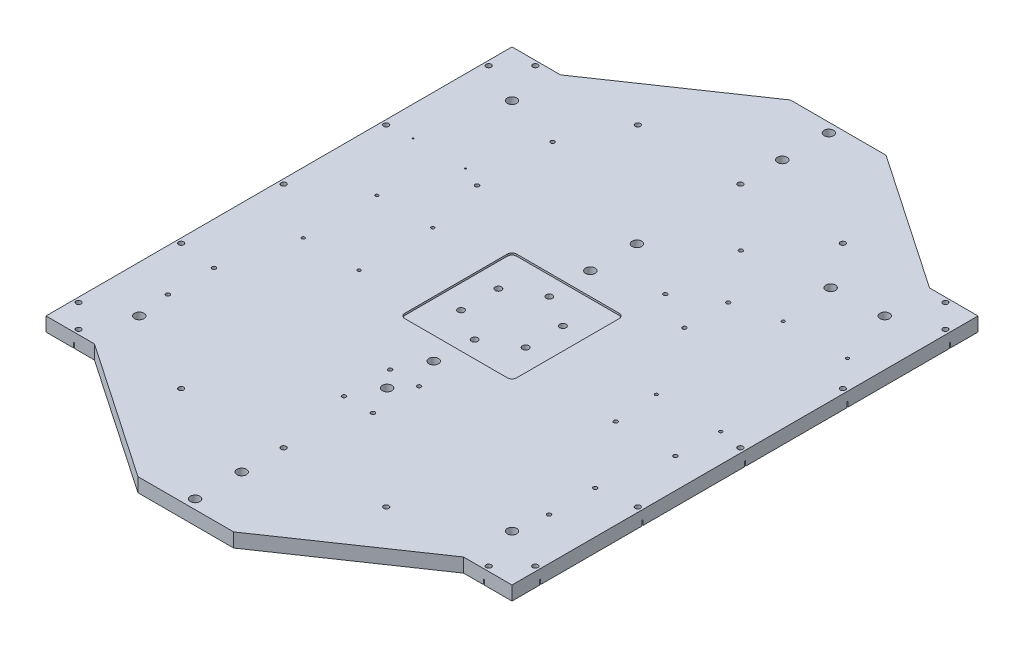
from build123d import *

# Parameters (mm, degrees)
SKETCH_5_W                     = 500
SKETCH_5_H                     = 500
EXTRUDE_1_DEPTH                = 15
EXTRUDE_2_DEPTH                = 60
EXTRUDE_3_DEPTH                = 60
HOLE_WIZARD_M8_1_D             = 6.8
HOLE_WIZARD_10_2_10_2_2_D      = 10.2
HOLE_WIZARD_M5_2_AT_2_COUNT    = 2
HOLE_WIZARD_M5_2_AT_2_PITCH    = 20
HOLE_WIZARD_M5_2_AT_3_COUNT    = 2
HOLE_WIZARD_M5_2_AT_3_PITCH    = 44.72135955
HOLE_WIZARD_M5_2_AT_4_COUNT    = 2
HOLE_WIZARD_M5_2_AT_4_PITCH    = 40
HOLE_WIZARD_M5_1_AT_2_COUNT    = 2
HOLE_WIZARD_M5_1_AT_2_PITCH    = 20
HOLE_WIZARD_M5_1_AT_3_COUNT    = 2
HOLE_WIZARD_M5_1_AT_3_PITCH    = 44.72135955
HOLE_WIZARD_M5_1_AT_4_COUNT    = 2
HOLE_WIZARD_M5_1_AT_4_PITCH    = 40
HOLE_WIZARD_10_2_10_2_1_D      = 10.2
HOLE_WIZARD_M5_3_D             = 4.2
HOLE_WIZARD_M5_4_D             = 4.2
HOLE_WIZARD_M4_1_D             = 3.3
HOLE_WIZARD_M2_1_D             = 1.6
HOLE_WIZARD_M12_3_D            = 10.2
HOLE_WIZARD_M3_5_1_D           = 2.9
HOLE_WIZARD_M3_5_1_DEPTH       = 10
SKETCH_47_W                    = 120
SKETCH_47_H                    = 120
CUT_EXTRUDE_1_DEPTH            = 2
CUT_EXTRUDE_2_DEPTH            = 60
CUT_EXTRUDE_3_DEPTH            = 460.292934847
HOLE_WIZARD_M5_1_2_D           = 5.5
HOLE_WIZARD_M5_1_2_CBORE_D     = 10.1
HOLE_WIZARD_M5_1_2_CBORE_DEPTH = 5.4
FILLET_1_R                     = 5


with BuildPart() as part:
    # 草图5 → 凸台-拉伸1 (new body)
    with BuildSketch(Plane(origin=(0, 0, 0), x_dir=(1, 0, 0), z_dir=(0, 1, 0))):
        Polygon((0, 385), (-198, 250), (198, 250), align=None)
        Rectangle(SKETCH_5_W, SKETCH_5_H)
        Polygon((198, -250), (-198, -250), (0, -385), align=None)
    extrude(amount=EXTRUDE_1_DEPTH)

    # 草图6 → 凸台-拉伸2 (add)
    with BuildSketch(Plane(origin=(0, 15, 0), x_dir=(1, 0, 0), z_dir=(0, 1, 0))):
        Polygon((198, 250), (0, 385), (-198, 250), (-250, 250), (-250, -250), (-198, -250), (0, -385), (198, -250), (250, -250), (250, 250), align=None)
        Polygon((-240, 240), (-240, -240), (-194.915297392, -240), (0, -372.896793677), (194.915297392, -240), (240, -240), (240, 240), (194.915297392, 240), (0, 372.896793677), (-194.915297392, 240), align=None, mode=Mode.SUBTRACT)
    extrude(amount=EXTRUDE_2_DEPTH)

    # 草图16 → 凸台-拉伸3 (add)
    with BuildSketch(Plane(origin=(0, 15, 0), x_dir=(1, 0, 0), z_dir=(0, 1, 0))):
        Polygon((180.248630726, -250), (194.915297392, -240), (-194.915297392, -240), (-180.248630726, -250), align=None)
        Polygon((-180.248630726, 250), (-194.915297392, 240), (194.915297392, 240), (180.248630726, 250), align=None)
    extrude(amount=EXTRUDE_3_DEPTH)

    # M8 螺纹孔1 (through all)
    with Locations(Plane(origin=(0, 15, -40), x_dir=(0, 0, 1), z_dir=(0, 1, 0))):
        with Locations((0, 0), (20, -34.641016151), (20, 34.641016151), (60, 34.641016151), (60, -34.641016151), (80, 0)):
            Hole(HOLE_WIZARD_M8_1_D / 2)

    # Ø10.2 (10.2) 直径孔2 (through all)
    with Locations(Plane(origin=(0, 15, -290), x_dir=(0, 0, 1), z_dir=(0, 1, 0))):
        with Locations((0, 0), (-50, 0), (156, 0), (206, 0)):
            hole_wizard_10_2_10_2_2 = Hole(HOLE_WIZARD_10_2_10_2_2_D / 2)

    # 镜向1: Ø10.2 (10.2) 直径孔2 across plane
    add(hole_wizard_10_2_10_2_2.mirror(Plane.XY), mode=Mode.SUBTRACT)

    # 草图22 → M5 螺纹孔2 (revolve, cut)
    with BuildSketch(Plane(origin=(214, 57.5, 250), x_dir=(0, -1, 0), z_dir=(1, 0, 0))):
        Polygon((0, 0), (0, 15.2618073), (2.1, 14), (2.1, 0), align=None)
    hole_wizard_m5_2 = revolve(axis=Axis((214, 57.5, 256.35), (0, 0, -1)), mode=Mode.SUBTRACT)

    # M5 螺纹孔2 at 2: M5 螺纹孔2 ×2
    with Locations(*[(i * HOLE_WIZARD_M5_2_AT_2_PITCH, 0, 0) for i in range(1, HOLE_WIZARD_M5_2_AT_2_COUNT)]):
        add(hole_wizard_m5_2, mode=Mode.SUBTRACT)

    # M5 螺纹孔2 at 3: M5 螺纹孔2 ×2
    with Locations(*[Vector(0.447213595499958, -0.894427190999916, 0) * (i * HOLE_WIZARD_M5_2_AT_3_PITCH) for i in range(1, HOLE_WIZARD_M5_2_AT_3_COUNT)]):
        add(hole_wizard_m5_2, mode=Mode.SUBTRACT)

    # M5 螺纹孔2 at 4: M5 螺纹孔2 ×2
    with Locations(*[(0, -i * HOLE_WIZARD_M5_2_AT_4_PITCH, 0) for i in range(1, HOLE_WIZARD_M5_2_AT_4_COUNT)]):
        add(hole_wizard_m5_2, mode=Mode.SUBTRACT)

    # 镜向2: M5 螺纹孔2 across plane
    add(hole_wizard_m5_2.mirror(Plane(origin=(0, 0, 0), x_dir=(0, 0, 1), z_dir=(1, 0, 0))), mode=Mode.SUBTRACT)

    # 镜向2 copy 1 sketch → 镜向2 copy 1 (revolve, cut)
    with BuildSketch(Plane(origin=(-234, 57.5, 250), x_dir=(0, -1, 0), z_dir=(-1, 0, 0))):
        Polygon((0, 0), (0, -15.2618073), (2.1, -14), (2.1, 0), align=None)
    revolve(axis=Axis((-234, 57.5, 256.35), (0, 0, 1)), mode=Mode.SUBTRACT)

    # 镜向2 copy 2 sketch → 镜向2 copy 2 (revolve, cut)
    with BuildSketch(Plane(origin=(-234, 17.5, 250), x_dir=(0, -1, 0), z_dir=(-1, 0, 0))):
        Polygon((0, 0), (0, -15.2618073), (2.1, -14), (2.1, 0), align=None)
    revolve(axis=Axis((-234, 17.5, 256.35), (0, 0, 1)), mode=Mode.SUBTRACT)

    # 镜向2 copy 3 sketch → 镜向2 copy 3 (revolve, cut)
    with BuildSketch(Plane(origin=(-214, 17.5, 250), x_dir=(0, -1, 0), z_dir=(-1, 0, 0))):
        Polygon((0, 0), (0, -15.2618073), (2.1, -14), (2.1, 0), align=None)
    revolve(axis=Axis((-214, 17.5, 256.35), (0, 0, 1)), mode=Mode.SUBTRACT)

    # 镜向3: M5 螺纹孔2 across plane
    add(hole_wizard_m5_2.mirror(Plane.XY), mode=Mode.SUBTRACT)

    # 镜向3 copy 1 sketch → 镜向3 copy 1 (revolve, cut)
    with BuildSketch(Plane(origin=(234, 57.5, -250), x_dir=(0, -1, 0), z_dir=(1, 0, 0))):
        Polygon((0, 0), (0, -15.2618073), (2.1, -14), (2.1, 0), align=None)
    revolve(axis=Axis((234, 57.5, -256.35), (0, 0, -1)), mode=Mode.SUBTRACT)

    # 镜向3 copy 2 sketch → 镜向3 copy 2 (revolve, cut)
    with BuildSketch(Plane(origin=(234, 17.5, -250), x_dir=(0, -1, 0), z_dir=(1, 0, 0))):
        Polygon((0, 0), (0, -15.2618073), (2.1, -14), (2.1, 0), align=None)
    revolve(axis=Axis((234, 17.5, -256.35), (0, 0, -1)), mode=Mode.SUBTRACT)

    # 镜向3 copy 3 sketch → 镜向3 copy 3 (revolve, cut)
    with BuildSketch(Plane(origin=(214, 17.5, -250), x_dir=(0, -1, 0), z_dir=(1, 0, 0))):
        Polygon((0, 0), (0, -15.2618073), (2.1, -14), (2.1, 0), align=None)
    revolve(axis=Axis((214, 17.5, -256.35), (0, 0, -1)), mode=Mode.SUBTRACT)

    # 镜向4 copy 1 sketch → 镜向4 copy 1 (revolve, cut)
    with BuildSketch(Plane(origin=(-214, 57.5, -250), x_dir=(0, -1, 0), z_dir=(-1, 0, 0))):
        Polygon((0, 0), (0, 15.2618073), (2.1, 14), (2.1, 0), align=None)
    revolve(axis=Axis((-214, 57.5, -256.35), (0, 0, 1)), mode=Mode.SUBTRACT)

    # 镜向4 copy 2 sketch → 镜向4 copy 2 (revolve, cut)
    with BuildSketch(Plane(origin=(-234, 57.5, -250), x_dir=(0, -1, 0), z_dir=(-1, 0, 0))):
        Polygon((0, 0), (0, 15.2618073), (2.1, 14), (2.1, 0), align=None)
    revolve(axis=Axis((-234, 57.5, -256.35), (0, 0, 1)), mode=Mode.SUBTRACT)

    # 镜向4 copy 3 sketch → 镜向4 copy 3 (revolve, cut)
    with BuildSketch(Plane(origin=(-234, 17.5, -250), x_dir=(0, -1, 0), z_dir=(-1, 0, 0))):
        Polygon((0, 0), (0, 15.2618073), (2.1, 14), (2.1, 0), align=None)
    revolve(axis=Axis((-234, 17.5, -256.35), (0, 0, 1)), mode=Mode.SUBTRACT)

    # 镜向4 copy 4 sketch → 镜向4 copy 4 (revolve, cut)
    with BuildSketch(Plane(origin=(-214, 17.5, -250), x_dir=(0, -1, 0), z_dir=(-1, 0, 0))):
        Polygon((0, 0), (0, 15.2618073), (2.1, 14), (2.1, 0), align=None)
    revolve(axis=Axis((-214, 17.5, -256.35), (0, 0, 1)), mode=Mode.SUBTRACT)

    # 镜向4 copy 5 sketch → 镜向4 copy 5 (revolve, cut)
    with BuildSketch(Plane(origin=(-214, 57.5, 250), x_dir=(0, -1, 0), z_dir=(-1, 0, 0))):
        Polygon((0, 0), (0, -15.2618073), (2.1, -14), (2.1, 0), align=None)
    revolve(axis=Axis((-214, 57.5, 256.35), (0, 0, 1)), mode=Mode.SUBTRACT)

    # 镜向4 copy 6 sketch → 镜向4 copy 6 (revolve, cut)
    with BuildSketch(Plane(origin=(-234, 57.5, 250), x_dir=(0, -1, 0), z_dir=(-1, 0, 0))):
        Polygon((0, 0), (0, -15.2618073), (2.1, -14), (2.1, 0), align=None)
    revolve(axis=Axis((-234, 57.5, 256.35), (0, 0, 1)), mode=Mode.SUBTRACT)

    # 镜向4 copy 7 sketch → 镜向4 copy 7 (revolve, cut)
    with BuildSketch(Plane(origin=(-234, 17.5, 250), x_dir=(0, -1, 0), z_dir=(-1, 0, 0))):
        Polygon((0, 0), (0, -15.2618073), (2.1, -14), (2.1, 0), align=None)
    revolve(axis=Axis((-234, 17.5, 256.35), (0, 0, 1)), mode=Mode.SUBTRACT)

    # 镜向4 copy 8 sketch → 镜向4 copy 8 (revolve, cut)
    with BuildSketch(Plane(origin=(-214, 17.5, 250), x_dir=(0, -1, 0), z_dir=(-1, 0, 0))):
        Polygon((0, 0), (0, -15.2618073), (2.1, -14), (2.1, 0), align=None)
    revolve(axis=Axis((-214, 17.5, 256.35), (0, 0, 1)), mode=Mode.SUBTRACT)

    # 草图25 → Hole Wizard M5 _1 (revolve, cut)
    with BuildSketch(Plane(origin=(-250, 57.5, -234), x_dir=(0, 0, 1), z_dir=(0, 1, 0))):
        Polygon((0, 0), (0, 15.2618073), (2.1, 14), (2.1, 0), align=None)
    hole_wizard_m5_1 = revolve(axis=Axis((-256.35, 57.5, -234), (1, 0, 0)), mode=Mode.SUBTRACT)

    # Hole Wizard M5 _1 at 2: Hole Wizard M5 _1 ×2
    with Locations(*[(0, 0, i * HOLE_WIZARD_M5_1_AT_2_PITCH) for i in range(1, HOLE_WIZARD_M5_1_AT_2_COUNT)]):
        add(hole_wizard_m5_1, mode=Mode.SUBTRACT)

    # Hole Wizard M5 _1 at 3: Hole Wizard M5 _1 ×2
    with Locations(*[Vector(0, -0.894427190999916, 0.447213595499958) * (i * HOLE_WIZARD_M5_1_AT_3_PITCH) for i in range(1, HOLE_WIZARD_M5_1_AT_3_COUNT)]):
        add(hole_wizard_m5_1, mode=Mode.SUBTRACT)

    # Hole Wizard M5 _1 at 4: Hole Wizard M5 _1 ×2
    with Locations(*[(0, -i * HOLE_WIZARD_M5_1_AT_4_PITCH, 0) for i in range(1, HOLE_WIZARD_M5_1_AT_4_COUNT)]):
        add(hole_wizard_m5_1, mode=Mode.SUBTRACT)

    # 镜向5: Hole Wizard M5 _1 across plane
    add(hole_wizard_m5_1.mirror(Plane.XY), mode=Mode.SUBTRACT)

    # 镜向5 copy 1 sketch → 镜向5 copy 1 (revolve, cut)
    with BuildSketch(Plane(origin=(-250, 57.5, 214), x_dir=(0, 0, -1), z_dir=(0, 1, 0))):
        Polygon((0, 0), (0, -15.2618073), (2.1, -14), (2.1, 0), align=None)
    revolve(axis=Axis((-256.35, 57.5, 214), (-1, 0, 0)), mode=Mode.SUBTRACT)

    # 镜向5 copy 2 sketch → 镜向5 copy 2 (revolve, cut)
    with BuildSketch(Plane(origin=(-250, 17.5, 214), x_dir=(0, 0, -1), z_dir=(0, 1, 0))):
        Polygon((0, 0), (0, -15.2618073), (2.1, -14), (2.1, 0), align=None)
    revolve(axis=Axis((-256.35, 17.5, 214), (-1, 0, 0)), mode=Mode.SUBTRACT)

    # 镜向5 copy 3 sketch → 镜向5 copy 3 (revolve, cut)
    with BuildSketch(Plane(origin=(-250, 17.5, 234), x_dir=(0, 0, -1), z_dir=(0, 1, 0))):
        Polygon((0, 0), (0, -15.2618073), (2.1, -14), (2.1, 0), align=None)
    revolve(axis=Axis((-256.35, 17.5, 234), (-1, 0, 0)), mode=Mode.SUBTRACT)

    # 镜向6: Hole Wizard M5 _1 across plane
    add(hole_wizard_m5_1.mirror(Plane(origin=(0, 0, 0), x_dir=(0, 0, 1), z_dir=(1, 0, 0))), mode=Mode.SUBTRACT)

    # 镜向6 copy 1 sketch → 镜向6 copy 1 (revolve, cut)
    with BuildSketch(Plane(origin=(250, 57.5, -214), x_dir=(0, 0, 1), z_dir=(0, 1, 0))):
        Polygon((0, 0), (0, -15.2618073), (2.1, -14), (2.1, 0), align=None)
    revolve(axis=Axis((256.35, 57.5, -214), (1, 0, 0)), mode=Mode.SUBTRACT)

    # 镜向6 copy 2 sketch → 镜向6 copy 2 (revolve, cut)
    with BuildSketch(Plane(origin=(250, 17.5, -214), x_dir=(0, 0, 1), z_dir=(0, 1, 0))):
        Polygon((0, 0), (0, -15.2618073), (2.1, -14), (2.1, 0), align=None)
    revolve(axis=Axis((256.35, 17.5, -214), (1, 0, 0)), mode=Mode.SUBTRACT)

    # 镜向6 copy 3 sketch → 镜向6 copy 3 (revolve, cut)
    with BuildSketch(Plane(origin=(250, 17.5, -234), x_dir=(0, 0, 1), z_dir=(0, 1, 0))):
        Polygon((0, 0), (0, -15.2618073), (2.1, -14), (2.1, 0), align=None)
    revolve(axis=Axis((256.35, 17.5, -234), (1, 0, 0)), mode=Mode.SUBTRACT)

    # 镜向6 copy 4 sketch → 镜向6 copy 4 (revolve, cut)
    with BuildSketch(Plane(origin=(250, 57.5, 234), x_dir=(0, 0, -1), z_dir=(0, 1, 0))):
        Polygon((0, 0), (0, 15.2618073), (2.1, 14), (2.1, 0), align=None)
    revolve(axis=Axis((256.35, 57.5, 234), (-1, 0, 0)), mode=Mode.SUBTRACT)

    # 镜向6 copy 5 sketch → 镜向6 copy 5 (revolve, cut)
    with BuildSketch(Plane(origin=(250, 57.5, 214), x_dir=(0, 0, -1), z_dir=(0, 1, 0))):
        Polygon((0, 0), (0, 15.2618073), (2.1, 14), (2.1, 0), align=None)
    revolve(axis=Axis((256.35, 57.5, 214), (-1, 0, 0)), mode=Mode.SUBTRACT)

    # 镜向6 copy 6 sketch → 镜向6 copy 6 (revolve, cut)
    with BuildSketch(Plane(origin=(250, 17.5, 214), x_dir=(0, 0, -1), z_dir=(0, 1, 0))):
        Polygon((0, 0), (0, 15.2618073), (2.1, 14), (2.1, 0), align=None)
    revolve(axis=Axis((256.35, 17.5, 214), (-1, 0, 0)), mode=Mode.SUBTRACT)

    # 镜向6 copy 7 sketch → 镜向6 copy 7 (revolve, cut)
    with BuildSketch(Plane(origin=(250, 17.5, 234), x_dir=(0, 0, -1), z_dir=(0, 1, 0))):
        Polygon((0, 0), (0, 15.2618073), (2.1, 14), (2.1, 0), align=None)
    revolve(axis=Axis((256.35, 17.5, 234), (-1, 0, 0)), mode=Mode.SUBTRACT)

    # Ø10.2 (10.2) 直径孔1 (through all)
    with Locations(Plane(origin=(-200, 0, 200), x_dir=(0, 0, -1), z_dir=(0, -1, 0))):
        with Locations((0, 0), (0, 400), (400, 400), (400, 0)):
            Hole(HOLE_WIZARD_10_2_10_2_1_D / 2)

    # M5 螺纹孔3 (through all)
    with Locations(Plane(origin=(217.801656439, 15, 42.5), x_dir=(0, 0, 1), z_dir=(0, 1, 0))):
        with Locations((0, 0), (0, -64), (72.75, -13.301656439), (122.25, -13.301656439), (72.75, -202.301656439), (122.25, -202.301656439), (122.25, -233.301656439), (72.75, -233.301656439), (72.75, -422.301656439), (122.25, -422.301656439), (-124, -114.301656439), (-171, -114.301656439)):
            Hole(HOLE_WIZARD_M5_3_D / 2)

    # M5 螺纹孔4 (through all)
    with Locations(Plane(origin=(-140, 15, -183.5), x_dir=(0, 0, 1), z_dir=(0, 1, 0))):
        with Locations((0, 0), (81, 0), (0, 202), (81, 202)):
            Hole(HOLE_WIZARD_M5_4_D / 2)

    # M4 螺纹孔1 (through all)
    with Locations(Plane(origin=(-184.5, 15, -39.5), x_dir=(0, 0, 1), z_dir=(0, 1, 0))):
        with Locations((0, 0), (79, 0), (0, 60), (79, 60), (-101, 404), (-101, 335), (35, 404), (35, 335)):
            Hole(HOLE_WIZARD_M4_1_D / 2)

    # M2 螺纹孔1 (through all)
    with Locations(Plane(origin=(-218, 15, -112), x_dir=(0, 0, 1), z_dir=(0, 1, 0))):
        with Locations((0, 0), (0, 56)):
            Hole(HOLE_WIZARD_M2_1_D / 2)

    # M12 螺纹孔3 (through all)
    with Locations(Plane(origin=(144.75, 15, -197.157303083), x_dir=(0, 0, 1), z_dir=(0, 1, 0))):
        with Locations((0, 0)):
            Hole(HOLE_WIZARD_M12_3_D / 2)

    # M3.5 螺纹孔1
    with Locations(Plane(origin=(59, 59.25, 240), x_dir=(-1, 0, 0), z_dir=(0, 0, -1))):
        with Locations((0, 0), (118, 0)):
            Hole(HOLE_WIZARD_M3_5_1_D / 2, depth=HOLE_WIZARD_M3_5_1_DEPTH)

    # 草图47 → 切除-拉伸1 (cut)
    with BuildSketch(Plane(origin=(0, 15, 0), x_dir=(1, 0, 0), z_dir=(0, 1, 0))):
        Rectangle(SKETCH_47_W, SKETCH_47_H)
    extrude(amount=-CUT_EXTRUDE_1_DEPTH, mode=Mode.SUBTRACT)

    # 草图48 → 切除-拉伸2 (cut)
    with BuildSketch(Plane(origin=(0, 75, 0), x_dir=(1, 0, 0), z_dir=(0, 1, 0))):
        Polygon((198, 250), (0, 385), (-198, 250), (-250, 250), (-250, -250), (-198, -250), (0, -385), (198, -250), (250, -250), (250, 250), align=None)
    extrude(amount=-CUT_EXTRUDE_2_DEPTH, mode=Mode.SUBTRACT)

    # 草图49 → 切除-拉伸3 (cut, through all)
    with BuildSketch(Plane(origin=(0, 15, 0), x_dir=(1, 0, 0), z_dir=(0, 1, 0))):
        Polygon((0, 385), (-51.333333333, 350), (51.333333333, 350), align=None)
        Polygon((51.333333333, -350), (0, -385), (-51.333333333, -350), align=None)
    extrude(amount=-CUT_EXTRUDE_3_DEPTH, mode=Mode.SUBTRACT)

    # Hole Wizard M5 _1 2 (through all)
    with Locations(Plane(origin=(0, 0, 0), x_dir=(-1, 0, 0), z_dir=(0, -1, 0))):
        with Locations((-245, 0), (-245, 110), (-245, 220), (-245, -220), (-245, -110), (245, -110), (245, -220), (245, 220), (245, 110), (245, 0), (0, 245), (110, 245), (220, 245), (-220, 245), (-110, 245), (-110, -245), (-220, -245), (220, -245), (110, -245), (0, -245)):
            CounterBoreHole(HOLE_WIZARD_M5_1_2_D / 2, HOLE_WIZARD_M5_1_2_CBORE_D / 2, HOLE_WIZARD_M5_1_2_CBORE_DEPTH)

    # 圆角1
    fillet_1_edges = [part.edges().sort_by_distance(p)[0] for p in [
        (-60, 14, 60),
        (-60, 14, -60),
        (60, 14, -60),
        (60, 14, 60),
    ]]
    fillet(fillet_1_edges, radius=FILLET_1_R)


solid = part.part
